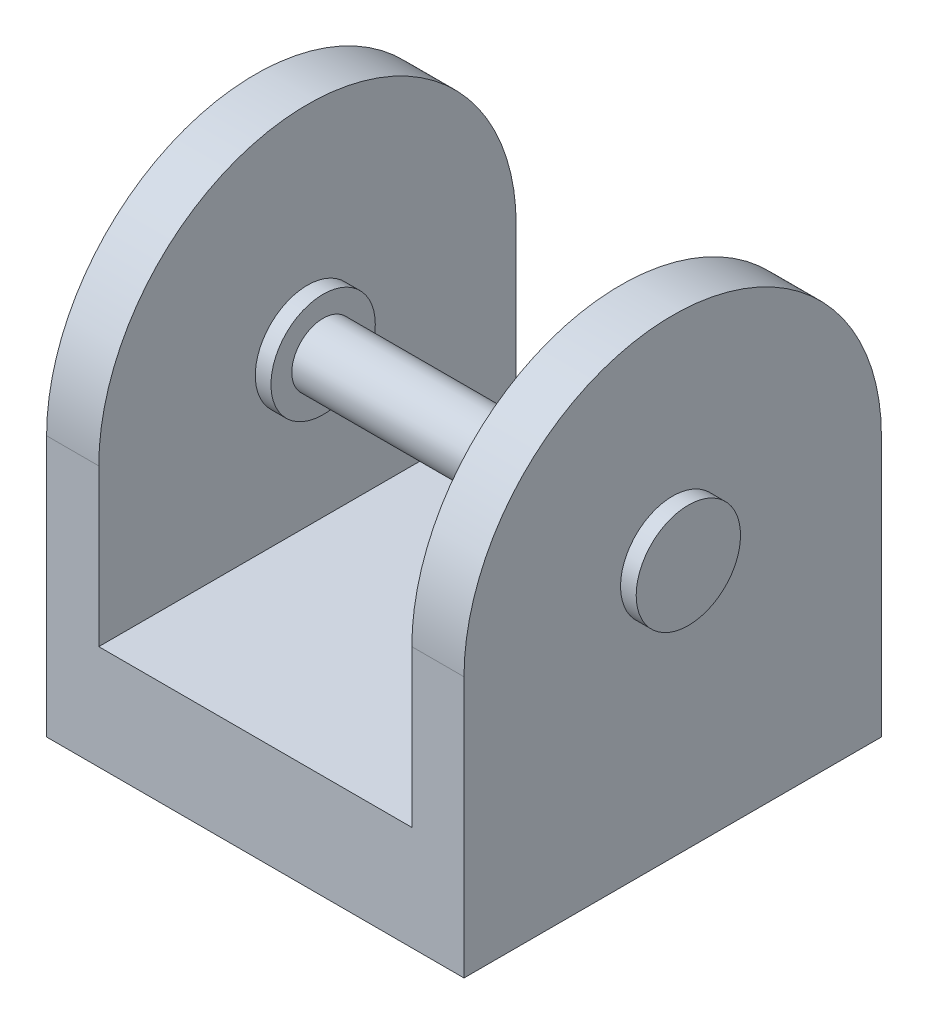
SolidWorks part; units mm, degrees
ref_plane "Front Plane" through (0, 0, 0) normal (0, 0, 1) x (1, 0, 0)
ref_plane "Top Plane" through (0, 0, 0) normal (0, 1, 0) x (1, 0, 0)
ref_plane "Right Plane" through (0, 0, 0) normal (1, 0, 0) x (0, 0, -1)
sketch "Sketch1" plane through (0, 0, 0) normal (0, 1, 0) x (1, 0, 0)
  line L1 (-20, 20) -> (20, 20)
  line L2 (-20, 20) -> (-20, -20)
  line L3 (-20, -20) -> (20, -20)
  line L4 (20, 20) -> (20, -20)
  line L5 (-20, 20) -> (20, -20) construction
  line L6 (-20, -20) -> (20, 20) construction
  point P0 (0, 0)
  dimension "D1" = 40
  dimension "D2" = 40
extrude "Boss-Extrude1" add sketch "Sketch1" along normal blind 10
sketch "Sketch2" plane through (20, 0, 0) normal (1, 0, 0) x (0, 0, -1)
  line L0 (0, 35.7483) -> (0, -19.103) construction
  line L5 (-20, 10) -> (-20, 25)
  line L6 (20, 10) -> (20, 25)
  line L7 (-20, 10) -> (20, 10)
  arc A0 (-20, 25) -> (20, 25) centre (0, 25) cw
  dimension "D1" = 15
extrude "Boss-Extrude2" add sketch "Sketch2" against normal blind 5
mirror "Mirror1" about plane through (0, 0, 0) normal (1, 0, 0) of "Boss-Extrude2"
ref_plane "Plane1" through (17.5, 0, 0) normal (1, 0, 0) x (0, 0, -1)
sketch "Sketch4" plane through (17.5, 0, 0) normal (1, 0, 0) x (0, 0, -1)
  circle A0 centre (0, 25) radius 5
  dimension "D1" = 10
extrude "Boss-Extrude3" add sketch "Sketch4" along normal mid plane 8
mirror "Mirror2" about plane through (0, 0, 0) normal (1, 0, 0) of "Boss-Extrude3"
sketch "Sketch5" plane through (13.5, 0, 0) normal (-1, 0, 0) x (0, 0, 1)
  circle A0 centre (0, 25) radius 3
  dimension "D1" = 6
extrude "Boss-Extrude4" add sketch "Sketch5" along normal up to next separate body
sketch "Sketch6" plane through (-21.5, 0, 0) normal (-1, 0, 0) x (0, 0, 1)
  circle A0 centre (0, 25) radius 5 construction
  circle A1 centre (0, 25) radius 5
extrude "Boss-Extrude5" add sketch "Sketch6" along normal blind 5
sketch "Sketch7" plane through (0, 0, 0) normal (0, -1, 0) x (1, 0, 0)
  circle A0 centre (0, 0) radius 3.4
  dimension "D1" = 6.8
